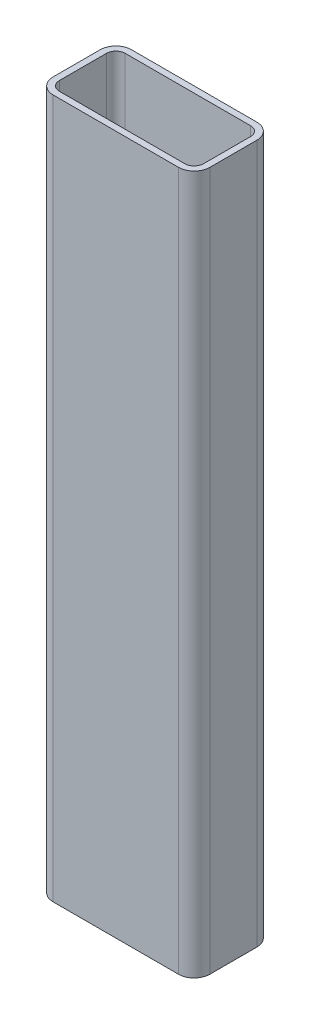
from build123d import *

# Parameters (mm, degrees)
EXTRUDE_THIN1_DEPTH = 223


with BuildPart() as part:
    # Sketch1 → Extrude-Thin1 (new, symmetric)
    with BuildSketch(Plane(origin=(0, 0, 0), x_dir=(1, 0, 0), z_dir=(0, 1, 0))):
        with BuildLine():
            Line((-40, 25), (40, 25))
            ThreePointArc((40, 25), (47.071067812, 22.071067812), (50, 15))
            Line((50, 15), (50, -15))
            ThreePointArc((50, -15), (47.071067812, -22.071067812), (40, -25))
            Line((40, -25), (-40, -25))
            ThreePointArc((-40, -25), (-47.071067812, -22.071067812), (-50, -15))
            Line((-50, -15), (-50, 15))
            ThreePointArc((-50, 15), (-47.071067812, 22.071067812), (-40, 25))
        make_face()
        with BuildLine():
            Line((-40, 21), (40, 21))
            ThreePointArc((40, 21), (44.242640687, 19.242640687), (46, 15))
            Line((46, 15), (46, -15))
            ThreePointArc((46, -15), (44.242640687, -19.242640687), (40, -21))
            Line((40, -21), (-40, -21))
            ThreePointArc((-40, -21), (-44.242640687, -19.242640687), (-46, -15))
            Line((-46, -15), (-46, 15))
            ThreePointArc((-46, 15), (-44.242640687, 19.242640687), (-40, 21))
        make_face(mode=Mode.SUBTRACT)
    extrude(amount=EXTRUDE_THIN1_DEPTH, both=True)


solid = part.part
